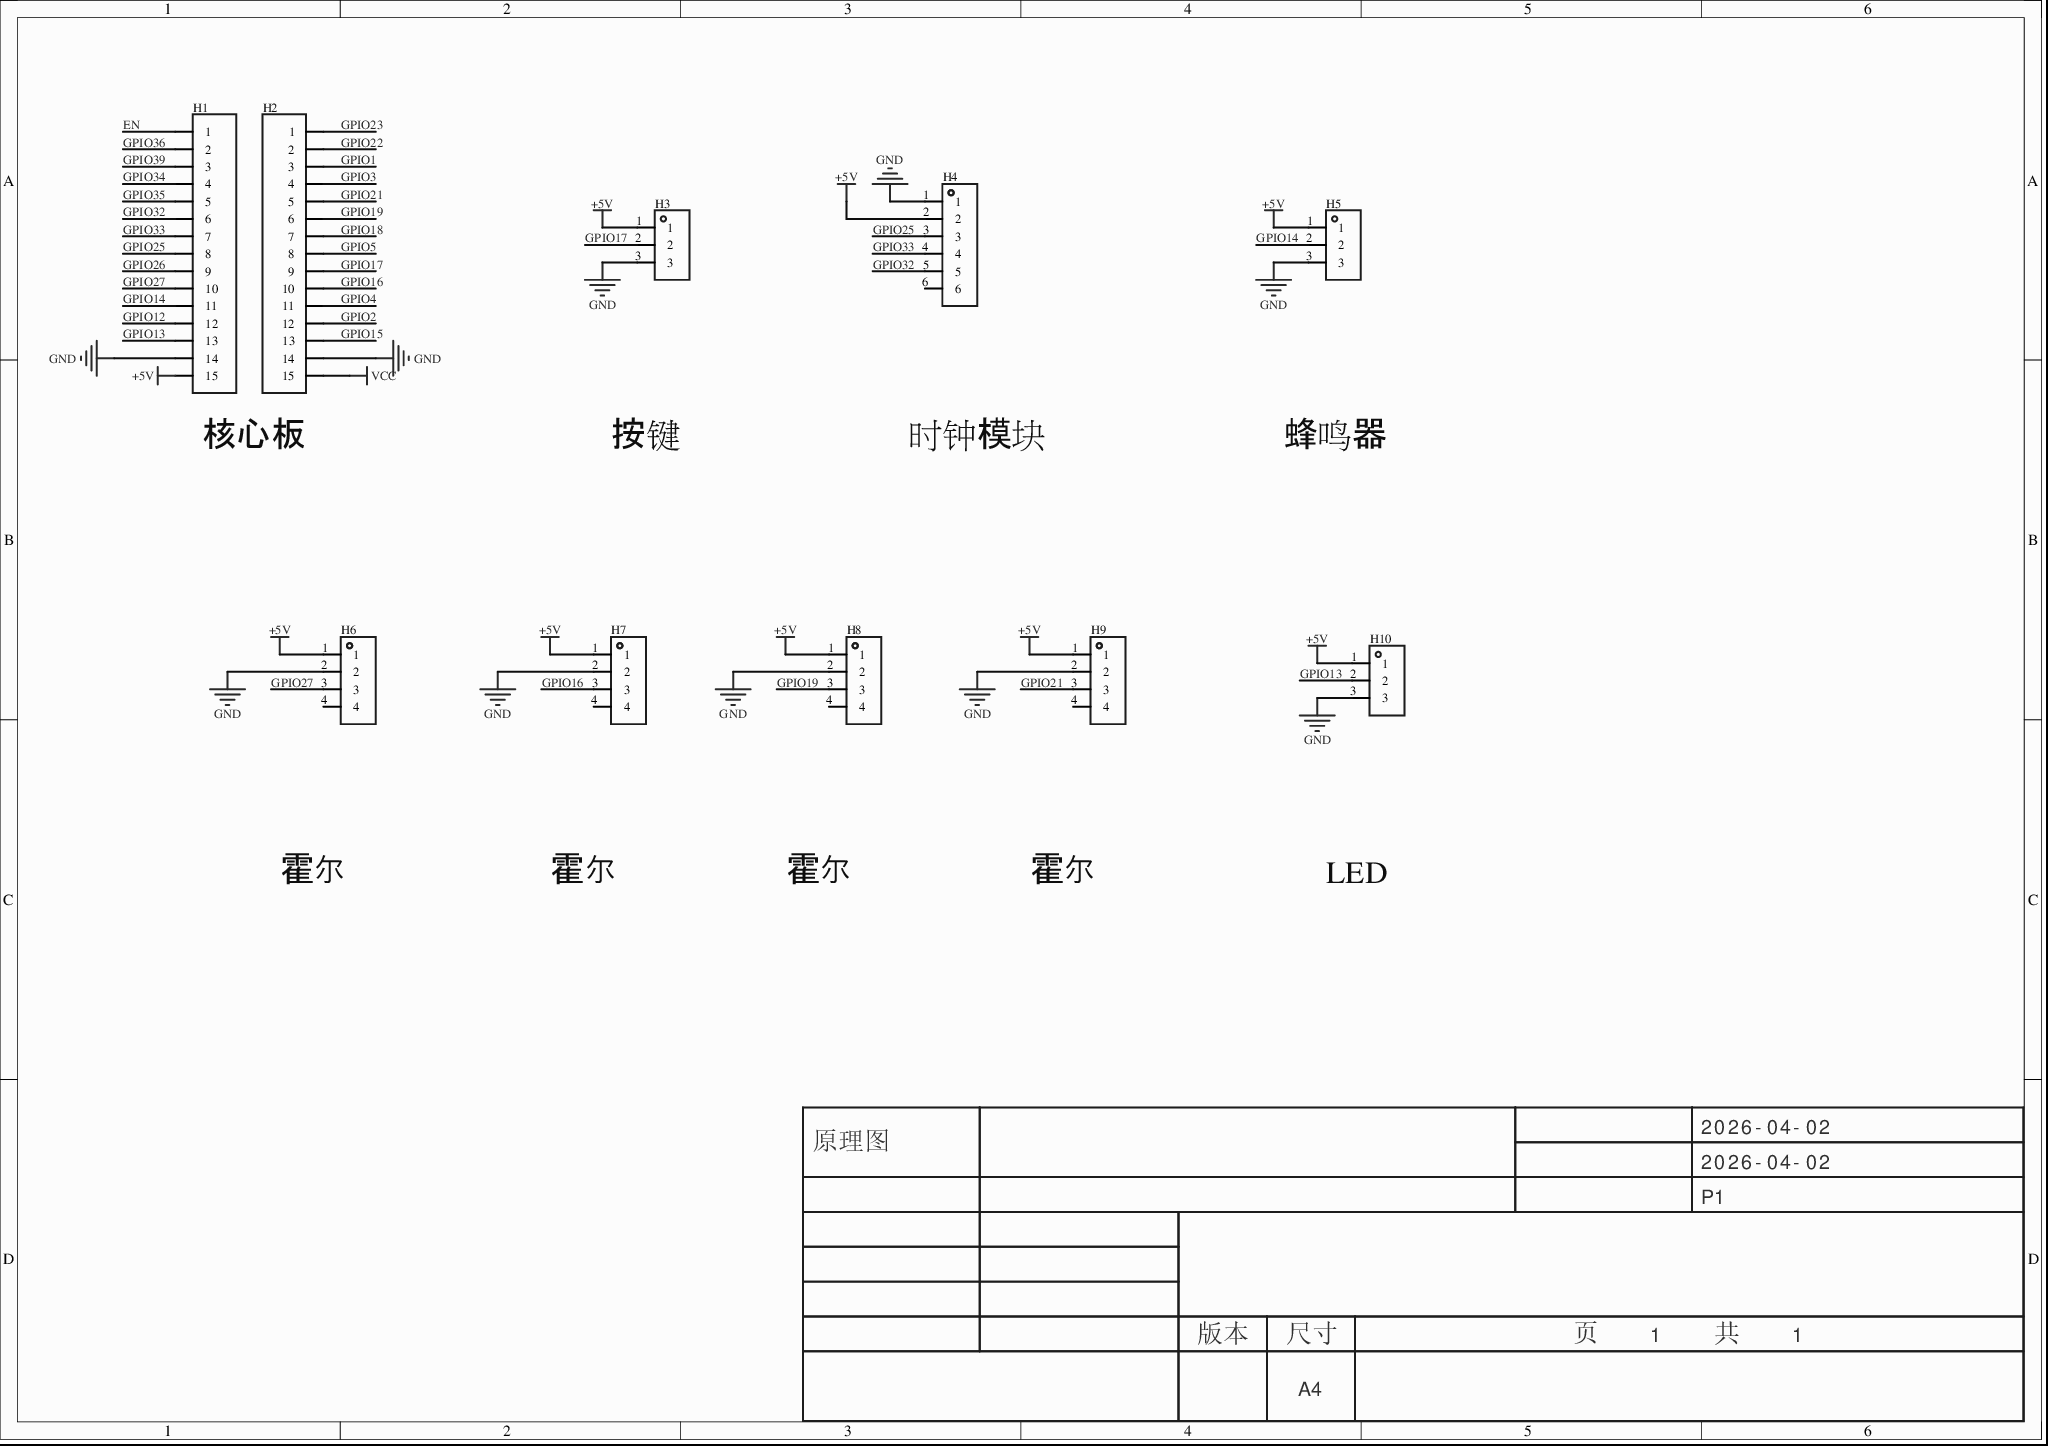
[diagram p0: MISC51778-3.schdoc]
# Altium project MISC51778-2.PrjPcb
1 sheet, 10 parts. Net scope: global (net labels, ports and power ports of the same name join across sheets).
Board file: MISC51778.pcbdoc

## Sheet MISC51778-3.schdoc
size 297 x 209 mm; Version: V1.0; @Project Name: MISC51778; @Update Date: 2026-04-02; @Create Date: 2026-04-02; @Board Name: MISC51778; @Create Time: 23:23:23; @Page Count: 1; @Page No: 1; @Schematic Name: MISC51778; @Update Time: 23:23:23; Size: A4

### Parts
H1  (no value)  [HDR-TH_15P-P2.54-V-F-1]
H2  (no value)  [HDR-TH_15P-P2.54-V-F-1]
H3  (no value)  [HDR-TH_3P-P2.54-V-F]
H4  (no value)  [HDR-TH_6P-P2.54-V-F]
H5  (no value)  [HDR-TH_3P-P2.54-V-F]
H6  (no value)  [HDR-TH_4P-P2.54-V-F]
H7  (no value)  [HDR-TH_4P-P2.54-V-F]
H8  (no value)  [HDR-TH_4P-P2.54-V-F]
H9  (no value)  [HDR-TH_4P-P2.54-V-F]
H10  (no value)  [HDR-TH_3P-P2.54-V-F]

### Nets
+5V: H1.15 H3.1 H4.2 H5.1 H6.1 H7.1 H8.1 H9.1 H10.1
GND: H1.14 H2.14 H3.3 H4.1 H5.3 H6.2 H7.2 H8.2 H9.2 H10.3
VCC: H2.15
EN: H1.1
GPIO1: H2.3
GPIO2: H2.12
GPIO3: H2.4
GPIO4: H2.11
GPIO5: H2.8
GPIO12: H1.12
GPIO13: H1.13 H10.2
GPIO14: H1.11 H5.2
GPIO15: H2.13
GPIO16: H2.10 H7.3
GPIO17: H2.9 H3.2
GPIO18: H2.7
GPIO19: H2.6 H8.3
GPIO21: H2.5 H9.3
GPIO22: H2.2
GPIO23: H2.1
GPIO25: H1.8 H4.3
GPIO26: H1.9
GPIO27: H1.10 H6.3
GPIO32: H1.6 H4.5
GPIO33: H1.7 H4.4
GPIO34: H1.4
GPIO35: H1.5
GPIO36: H1.2
GPIO39: H1.3

Not connected (* = marked no-connect by the designer): H4 6; H6 4; H7 4; H8 4; H9 4

### Notes on the sheet
- (near H1) 核心板
- 按键
- 时钟模块
- 蜂鸣器
- 霍尔
- LED
- 2026-04-02
- 原理图
- P1
- 版本
- 尺寸
- A4
- 页    1    共    1

### Library data of the parts
H1 H2 = HDR-F_2.54_1x15P: ConvertToPcb: yes; ModelId: 88d88d3d05774da49ce8fa2ce222e7100819f05c4eef4c71ace90d822a990e87; ModelTransform: 1515.745,94.488,0,0,0,0,0,0,-125.984; Symbol: HDR-F_2.54_1x15P; Device: HDR-F_2.54_1x15P; AddInBom: yes; SupplierPart: C124408; Supplier Footprint: 插件,; FootprintName: HDR-TH_15P-P2.54-V-F-1; ModelName: HDR-TH_15P-P2.54-V-F-1
H3 H5 H10 = HDR-F_2.54_1x3P: Symbol: PM254V-11-03-H85; ConvertToPcb: yes; ModelId: f3b3cc5aae9641bf9e56fc160cef875b0819f05c4eef4c71ace90d822a990e87; ModelName: HDR2.54-F-LI-1X3P; ModelTransform: 299.9994,100,0,0,0,0,0,0,-118.11; Device: HDR-F_2.54_1x3P; AddInBom: yes; SupplierPart: C541850; Supplier Footprint: 插件; FootprintName: HDR-TH_3P-P2.54-V-F
H4 = HDR-F_2.54_1x6P: Symbol: Header-Female-2.54_1x6; ConvertToPcb: yes; ModelId: 0f5bcf94dcda47d085f24cdca1696fe90819f05c4eef4c71ace90d822a990e87; ModelTransform: 619.684,94.488,0,0,0,0,0,0,-125.984; Device: HDR-F_2.54_1x6P; AddInBom: yes; SupplierPart: C40877; Supplier Footprint: 插件; FootprintName: HDR-TH_6P-P2.54-V-F; ModelName: HDR-TH_6P-P2.54-V-F
H6-H9 = HDR-F_2.54_1x4P: Symbol: 2.54-1*4P母; ConvertToPcb: yes; ModelId: d187812051054f85879fcaa51a310d8e0819f05c4eef4c71ace90d822a990e87; ModelTransform: 419.6842,98.464,0,0,0,0,0,0,-118.11; Device: HDR-F_2.54_1x4P; AddInBom: yes; SupplierPart: C2718488; Supplier Footprint: 插件; FootprintName: HDR-TH_4P-P2.54-V-F; ModelName: HDR-TH_4P-P2.54-V-F